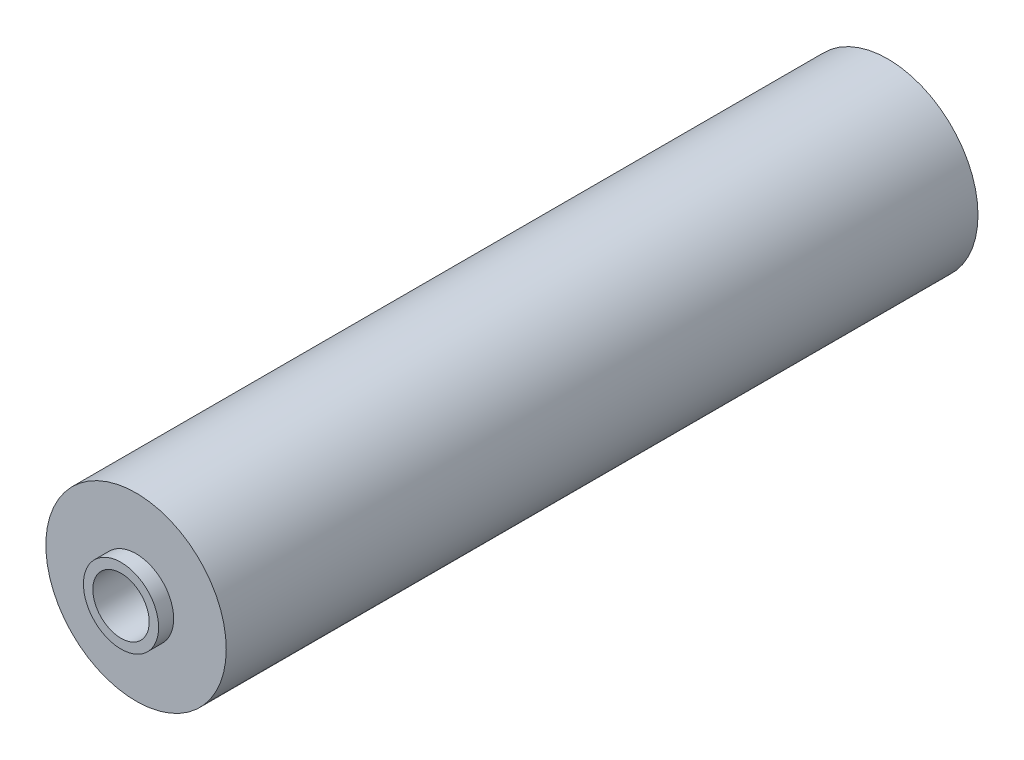
SolidWorks part; units mm, degrees
ref_plane "前视基准面" through (0, 0, 0) normal (0, 0, 1) x (1, 0, 0)
ref_plane "上视基准面" through (0, 0, 0) normal (0, 1, 0) x (1, 0, 0)
ref_plane "右视基准面" through (0, 0, 0) normal (1, 0, 0) x (0, 0, -1)
sketch "草图1" plane through (0, 0, 0) normal (0, 0, 1) x (1, 0, 0)
  circle A0 centre (0, 0) radius 120
  dimension "D1" = 240
extrude "凸台-拉伸1" add sketch "草图1" along normal blind 1000
sketch "草图2" plane through (0, 0, 1000) normal (0, 0, 1) x (1, 0, 0)
  circle A0 centre (0, 0) radius 37.5
  dimension "D1" = 75
extrude "切除-拉伸1" cut sketch "草图2" against normal blind 1000
sketch "草图3" plane through (0, 0, 1000) normal (0, 0, 1) x (1, 0, 0)
  circle A0 centre (0, 0) radius 50
  circle A1 centre (0, 0) radius 37.5
  dimension "D1" = 100
extrude "凸台-拉伸2" add sketch "草图3" along normal blind 20
ref_plane "基准面1" through (0, 0, 500) normal (0, 0, 1) x (1, 0, 0)
mirror "镜向1" about plane through (0, 0, 500) normal (0, 0, 1) of "凸台-拉伸2"
